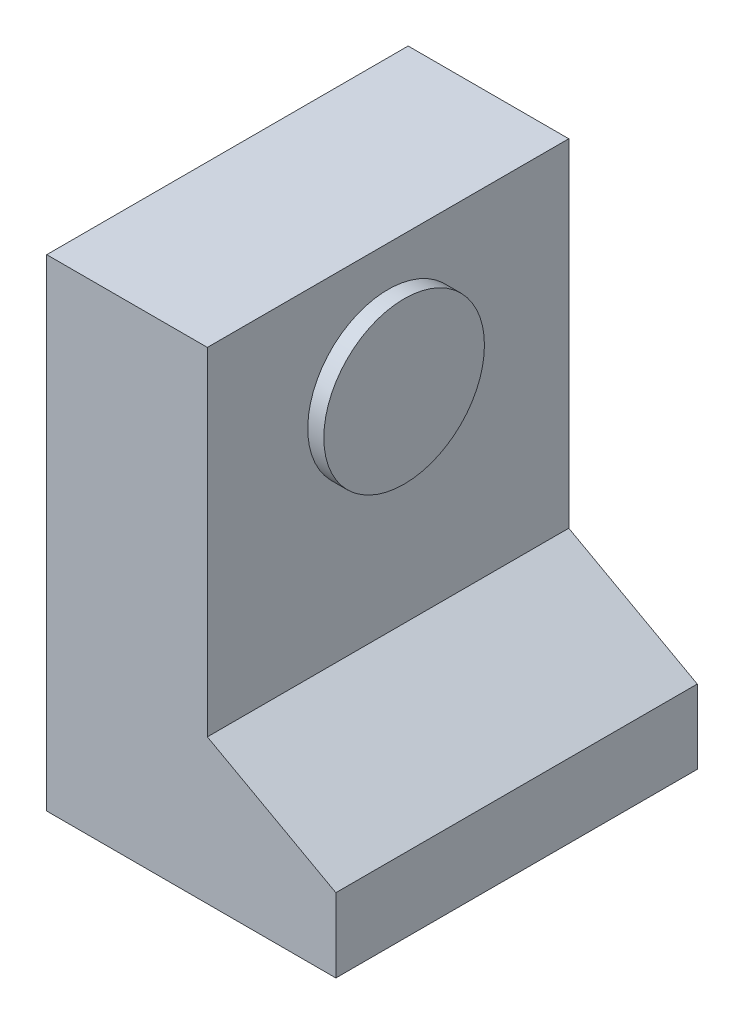
SolidWorks part; units mm, degrees
ref_plane "Front Plane" through (0, 0, 0) normal (0, 0, 1) x (1, 0, 0)
ref_plane "Top Plane" through (0, 0, 0) normal (0, 1, 0) x (1, 0, 0)
ref_plane "Right Plane" through (0, 0, 0) normal (1, 0, 0) x (0, 0, -1)
other "Configuration Table"
sketch "Sketch1" plane through (0, 0, 0) normal (1, 0, 0) x (0, 0, -1)
  line L1 (-225, 300) -> (225, 300)
  line L2 (-225, 300) -> (-225, -300)
  line L3 (-225, -300) -> (225, -300)
  line L4 (225, 300) -> (225, -300)
  line L5 (-225, 300) -> (225, -300) construction
  line L6 (-225, -300) -> (225, 300) construction
  point P0 (0, 0)
  dimension "D1" = 450
  dimension "D2" = 600
extrude "Boss-Extrude1" add sketch "Sketch1" along normal blind 400
sketch "Sketch2" plane through (0, 0, 225) normal (0, 0, 1) x (1, 0, 0)
  line L0 (400, 300) -> (0, 300) construction
  line L1 (200, 300) -> (200, -120)
  line L2 (200, -120) -> (400, -230)
  line L3 (400, 300) -> (400, -300) construction
  line L4 (400, -230) -> (400, 300)
  line L5 (400, 300) -> (200, 300)
  line L6 (400, -300) -> (0, -300) construction
  dimension "D1" = 200
  dimension "D2" = 420
  dimension "D3" = 70
extrude "Cut-Extrude1" cut sketch "Sketch2" against normal blind 2400
sketch "Sketch3" plane through (200, 0, 0) normal (1, 0, 0) x (0, 0, -1)
  line L0 (0, 300) -> (0, 0) construction
  line L1 (225, 300) -> (-225, 300) construction
  line L2 (-225, -300) -> (225, -300) construction
  circle A0 centre (0, 150) radius 100
  circle A1 centre (0, 150) radius 50
  dimension "D1" = 200
  dimension "D2" = 100
  dimension "D3" = 450
sketch "Sketch4" plane through (400, 0, 0) normal (1, 0, 0) x (0, 0, -1)
  line L1 (-326.8524, -171.5118) -> (321.9521, -171.5118)
  line L2 (-326.8524, -171.5118) -> (-326.8524, -354.7843)
  line L3 (-326.8524, -354.7843) -> (321.9521, -354.7843)
  line L4 (321.9521, -171.5118) -> (321.9521, -354.7843)
extrude "Cut-Extrude2" cut sketch "Sketch4" against normal blind 40
sketch "Sketch5" plane through (200, 0, 0) normal (1, 0, 0) x (0, 0, -1)
  circle A0 centre (0, 150) radius 100
extrude "Boss-Extrude2" add sketch "Sketch5" along normal blind 20
